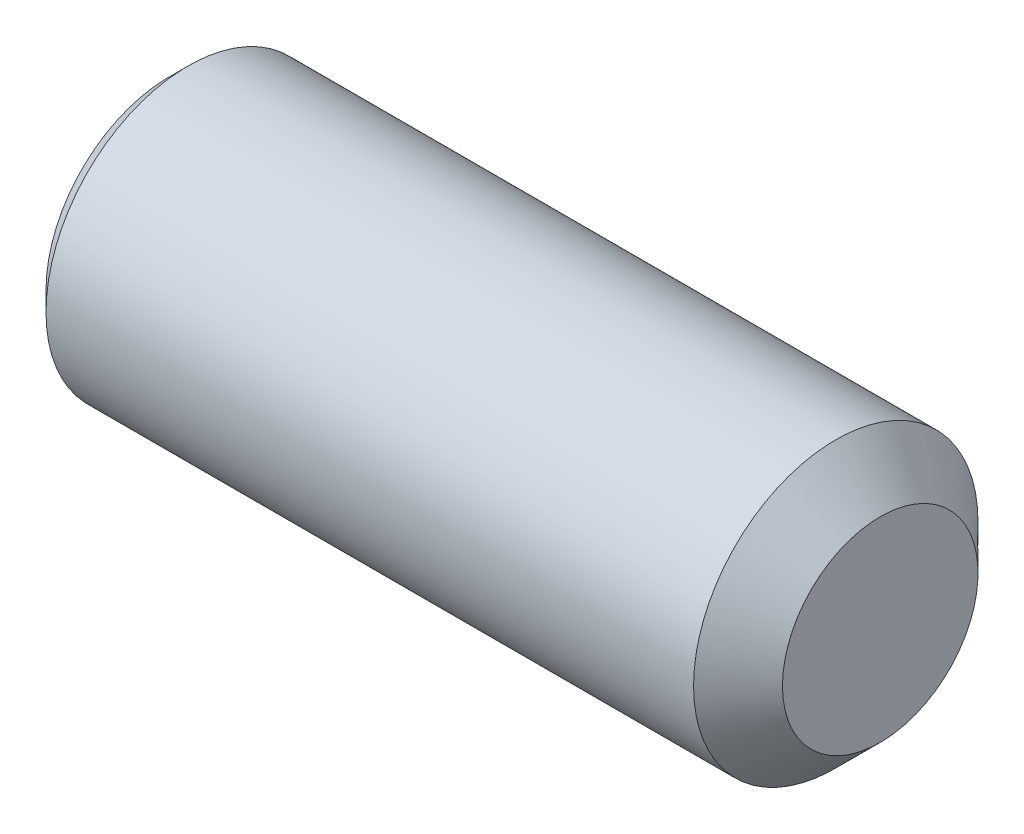
SolidWorks part; units mm, degrees
ref_plane "前视" through (0, 0, 0) normal (0, 0, 1) x (1, 0, 0)
ref_plane "上视" through (0, 0, 0) normal (0, 1, 0) x (1, 0, 0)
ref_plane "右视" through (0, 0, 0) normal (1, 0, 0) x (0, 0, -1)
sketch "尺寸草图" plane through (0, 0, 0) normal (0, 0, 1) x (1, 0, 0)
  line L0 (0, 0) -> (20, 0) construction
  point P3 (5, 0)
  point P4 (18.75, 0)
  point P5 (14.5, 0)
  point P6 (6.928, 0)
  point P7 (8, 0)
  point P8 (15.417, 0)
  point P9 (4, 0)
  dimension "l" = 20
  dimension "t" = 5
  dimension "P" = 1.25
  dimension "dp" = 5.5
  dimension "df" = 6.928
  dimension "d" = 8
  dimension "e" = 4.583
  dimension "s" = 4
sketch "草图1" plane through (0, 0, 0) normal (0, 0, 1) x (1, 0, 0)
  line L0 (0, 0) -> (20, 0)
  line L1 (20, 0) -> (20, 2.75)
  line L2 (20, 2.75) -> (18.75, 4)
  line L3 (18.75, 4) -> (0.536, 4)
  line L4 (0.536, 4) -> (0, 3.464)
  line L5 (0, 3.464) -> (0, 0)
  line L6 (-0.2778, 0) -> (5.1995, 0) construction
  dimension "D1" = 45
  dimension "l" = 20
  dimension "df" = 6.928
  dimension "d" = 8
  dimension "dp" = 5.5
  dimension "D2" = 45
revolve "基体-旋转" add sketch "草图1" angle 360 about L6
cosmetic thread "装饰螺纹线1" parameters "df"=6.928
sketch "草图2" plane through (0, 0, 0) normal (-1, 0, 0) x (0, 0, 1)
  line L1 (-1.1547, -2) -> (1.1547, -2)
  line L2 (1.1547, -2) -> (2.3094, 0)
  line L3 (2.3094, 0) -> (1.1547, 2)
  line L4 (1.1547, 2) -> (-1.1547, 2)
  line L5 (-1.1547, 2) -> (-2.3094, 0)
  line L6 (-2.3094, 0) -> (-1.1547, -2)
  circle A0 centre (0, 0) radius 2 construction
  dimension "D1" = 4
extrude "切除-拉伸1" cut sketch "草图2" against normal blind 5
sketch "草图4" plane through (0, 0, 0) normal (0, 0, 1) x (1, 0, 0)
  line L0 (-0.2778, 0) -> (1.1933, 0) construction
  line L2 (-0.2778, 0) -> (5.1995, 0) construction
  line L3 (5, 2) -> (6.1547, 0)
  line L4 (6.1547, 0) -> (5, 0)
  line L5 (5, 0) -> (5, 2)
  line L6 (5, 2) -> (0, 2) construction
  dimension "D1" = 60
  dimension "D2" = 5
revolve "切除-旋转2" cut sketch "草图4" angle 360 about L0
sketch "草图5" plane through (0, 0, 0) normal (0, 0, 1) x (1, 0, 0)
  line L0 (0.536, 4) -> (1.786, 4)
  line L1 (18.75, 4) -> (0.536, 4) construction
  line L2 (1.786, 4) -> (1.1542, 2.9175)
  line L3 (1.1542, 2.9175) -> (0.536, 4)
  line L5 (5.1995, 0) -> (3.6008, 0) construction
  line L6 (-0.2778, 0) -> (5.1995, 0) construction
  line L7 (0.536, 4) -> (0, 3.464) construction
  dimension "D1" = 1.0825
  dimension "P" = 1.25
  dimension "D2" = 60
revolve "切除-旋转3" [suppressed] cut sketch "草图5" angle 360 about L5
pattern_linear "阵列(线性)1" [suppressed] count 16
